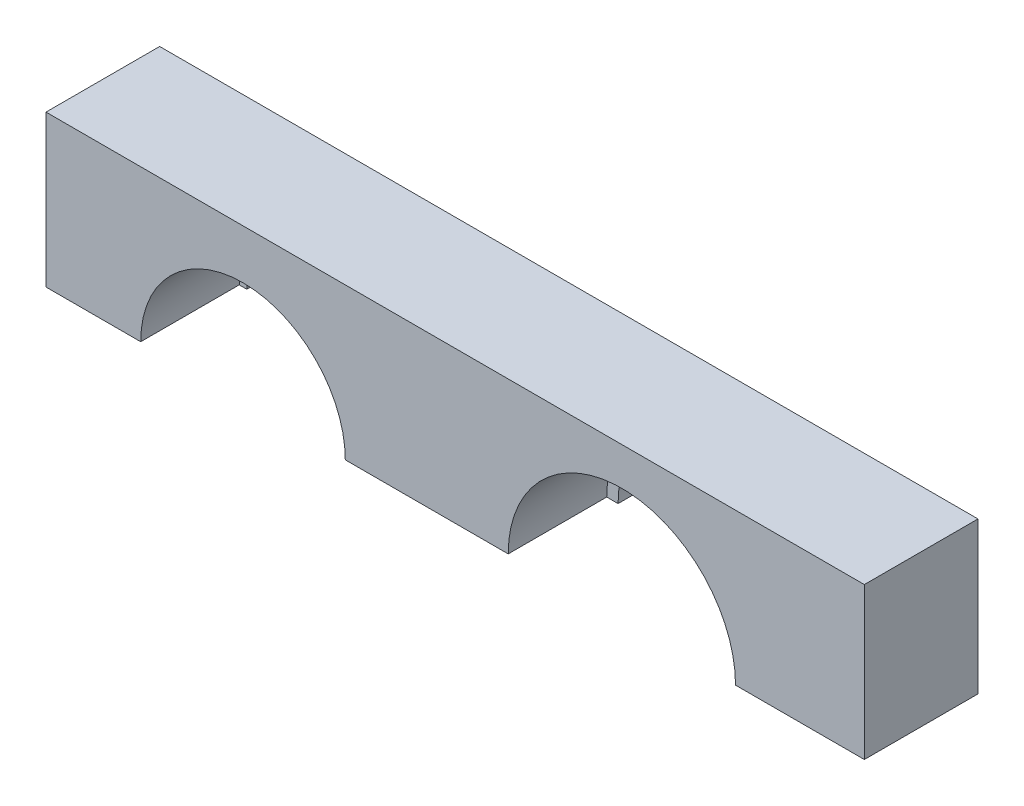
from build123d import *

# Parameters (mm, degrees)
SKETCH_1_W               = 1080
SKETCH_1_H               = 200
EXTRUDE_1_DEPTH          = 150
SKETCH_2_R               = 135
SKETCH_2_R_2             = 150
CUT_EXTRUDE_1_DEPTH      = 130
CUT_EXTRUDE_2_DEPTH      = 570.2978131
CUT_EXTRUDE_2_DEPTH_BACK = 570.2978131
SKETCH_2_3_R             = 125
SKETCH_2_3_R_2           = 135


with BuildPart() as part:
    # 草图1 → 凸台-拉伸1 (new body)
    with BuildSketch(Plane.XY):
        Rectangle(SKETCH_1_W, SKETCH_1_H)
    extrude(amount=EXTRUDE_1_DEPTH)

    # 草图2 → 切除-拉伸1 (cut)
    with BuildSketch(Plane.XY.offset(150)):
        with Locations((-280, -100)):
            Circle(SKETCH_2_R)
        with Locations((220, -100)):
            Circle(SKETCH_2_R_2)
    extrude(amount=-CUT_EXTRUDE_1_DEPTH, mode=Mode.SUBTRACT)

    # 草图2<3> → 切除-拉伸2 (cut, two sides: drawn at the far end of the back side and taken through both)
    with BuildSketch(Plane.XY.offset(150).offset(-CUT_EXTRUDE_2_DEPTH_BACK)):
        with Locations((-280, -100)):
            Circle(SKETCH_2_3_R)
        with Locations((220, -100)):
            Circle(SKETCH_2_3_R_2)
    extrude(amount=CUT_EXTRUDE_2_DEPTH + CUT_EXTRUDE_2_DEPTH_BACK, mode=Mode.SUBTRACT)


solid = part.part
